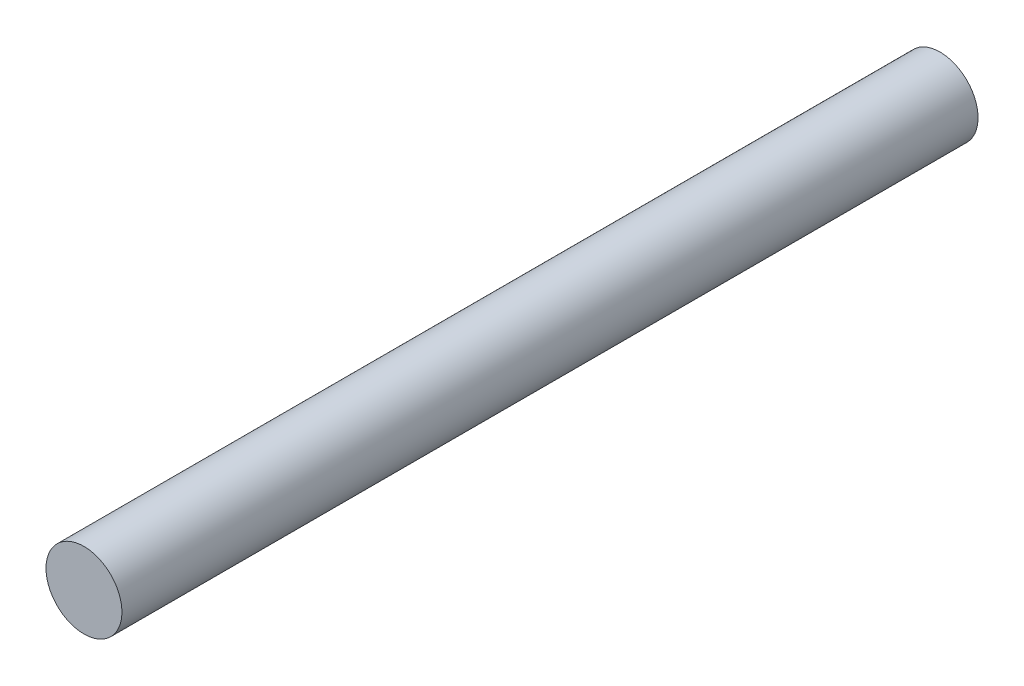
from build123d import *

# Parameters (mm, degrees)
BOSS_EXTRUDE1_DEPTH      = 38.1
BOSS_EXTRUDE1_DEPTH_BACK = 38.1
SKETCH2_R                = 3.3782


with BuildPart() as part:
    # Sketch2 → Boss-Extrude1 (new, two sides: drawn at the far end of the back side and taken through both)
    with BuildSketch(Plane.XY.offset(-BOSS_EXTRUDE1_DEPTH_BACK)):
        with Locations(Location((0, 0, 0), (0, 0, 180))):
            Circle(SKETCH2_R)
    extrude(amount=BOSS_EXTRUDE1_DEPTH + BOSS_EXTRUDE1_DEPTH_BACK)


solid = part.part
